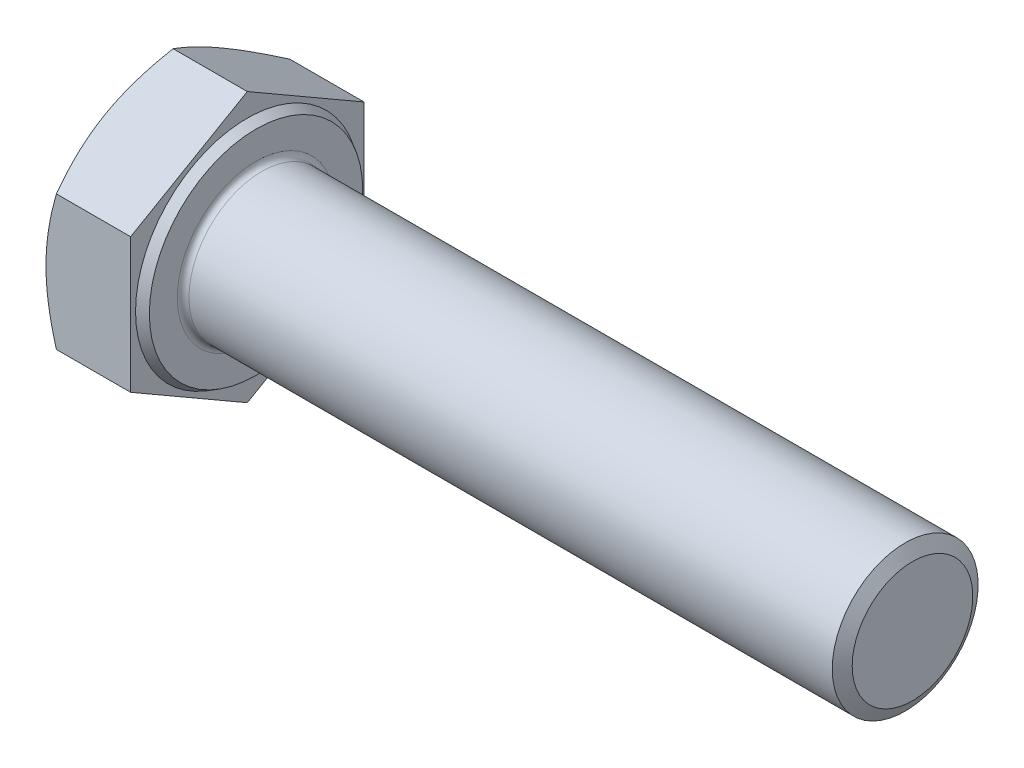
SolidWorks part; units mm, degrees
ref_plane "前视" through (0, 0, 0) normal (0, 0, 1) x (1, 0, 0)
ref_plane "上视" through (0, 0, 0) normal (0, 1, 0) x (1, 0, 0)
ref_plane "右视" through (0, 0, 0) normal (1, 0, 0) x (0, 0, -1)
sketch "草图1" plane through (0, 0, 0) normal (1, 0, 0) x (0, 0, -1)
  line L0 (8, 4.6188) -> (8, -4.6188)
  line L1 (-8, 4.6188) -> (-8, -4.6188)
  line L2 (8, -4.6188) -> (0, -9.2376)
  line L3 (0, -9.2376) -> (-8, -4.6188)
  line L4 (8, 4.6188) -> (0, 9.2376)
  line L5 (0, 9.2376) -> (-8, 4.6188)
  circle A0 centre (0, 0) radius 8.885 construction
  dimension "e" = 17.77
  dimension "s" = 16
  dimension "D2" = 120
  dimension "D3" = 8
  dimension "D4" = 8
  dimension "D5" = 8
extrude "基体-拉伸" add sketch "草图1" along normal blind 6.4
sketch "草图2" plane through (0, 0, 0) normal (0, 0, 1) x (1, 0, 0)
  line L0 (0, 4.6188) -> (0, -4.6188) construction
  line L1 (0, 0) -> (51.4, 0)
  line L2 (0, 0) -> (0, 5)
  line L3 (0, 5) -> (25.7, 5)
  line L4 (51.4, 0) -> (51.4, 4.134)
  line L5 (6.4, 9.2376) -> (6.4, 4.6188) construction
  line L6 (0, 0) -> (-11.2, 0) construction
  line L7 (0, 0) -> (96.52, 0) construction
  line L8 (51.4, -4.134) -> (25.7, -5) construction
  line L9 (0, -5) -> (25.7, -5) construction
  line L10 (7.4, 15.24) -> (7.4, -1.27) construction
  line L11 (25.4, 15.24) -> (25.4, -1.27) construction
  line L12 (6.4, 4.6188) -> (6.4, -4.6188) construction
  line L13 (25.7, 5) -> (51.4, 5)
  line L14 (51.4, 5) -> (51.4, 4.134)
  line L15 (-11.2, 0) -> (-11.2, 10) construction
  dimension "l" = 45
  dimension "d" = 10
  dimension "Minor_dia" = 8.268
  dimension "p" = 1
  dimension "b" = 26
  dimension "da" = 11.2
  dimension "ds" = 10
revolve "凸台-旋转1" add sketch "草图2" angle 360 about L7
cosmetic thread "螺旋线1" parameters "Thread_length"=26, "Thread_minor"=8.268
sketch "草图3" plane through (0, 0, 0) normal (0, 0, 1) x (1, 0, 0)
  line L0 (0, 8) -> (3.6013, 14.2376)
  line L1 (0, 9.2376) -> (0, 4.6188) construction
  line L2 (3.6013, 14.2376) -> (3.6013, 19.2376)
  line L3 (3.6013, 19.2376) -> (-10, 19.2376)
  line L4 (-10, 19.2376) -> (-10, 8)
  line L5 (-10, 8) -> (0, 8)
  line L6 (0, 0) -> (99.06, 0) construction
  line L7 (6.4, 9.2376) -> (0, 9.2376) construction
  dimension "D1" = 8
  dimension "D2" = 5
  dimension "D3" = 10
  dimension "D4" = 5
  dimension "Head_ch_ang" = 30
revolve "切除-旋转1" cut sketch "草图3" angle 360 about L6
sketch "草图4" plane through (0, 0, 0) normal (0, 0, 1) x (1, 0, 0)
  line L0 (0, 0) -> (216.8159, 0) construction
  line L2 (6.4, 0) -> (6.4, 7.315) construction
  line L9 (6.4, -5) -> (6.4, 5) construction
  line L10 (6.4, 9.2376) -> (6.4, 4.6188) construction
  line L11 (6.4, 7.315) -> (5.8, 7.6614)
  line L12 (5.8, 7.6614) -> (5.8, 9.2376)
  line L13 (6.4, 9.2376) -> (0.7145, 9.2376) construction
  line L14 (5.8, 9.2376) -> (6.4, 9.2376)
  line L15 (6.4, 9.2376) -> (6.4, 7.315)
  dimension "D1" = 120
  dimension "c" = 0.6
  dimension "dw" = 14.63
revolve "切除-旋转3" cut sketch "草图4" angle 360 about L0
fillet "圆角" radius 0.4 1 edges at (6.4, 0, -5)
sketch "草图6" plane through (0, 0, 0) normal (0, 0, 1) x (1, 0, 0)
  line L0 (0, 0) -> (51.4, 0) construction
  line L1 (51.4, -5) -> (51.4, 5) construction
  line L2 (51.4, 0) -> (51.4, 5) construction
  line L4 (50.9, 5) -> (51.9, 5)
  line L5 (50.9, 5) -> (51.4, 4.134)
  line L6 (51.4, 4.134) -> (51.9, 5)
  dimension "D1" = 1
revolve "切除-旋转4" cut sketch "草图6" angle 360 about L0
pattern_linear "阵列(线性)1" [suppressed]
